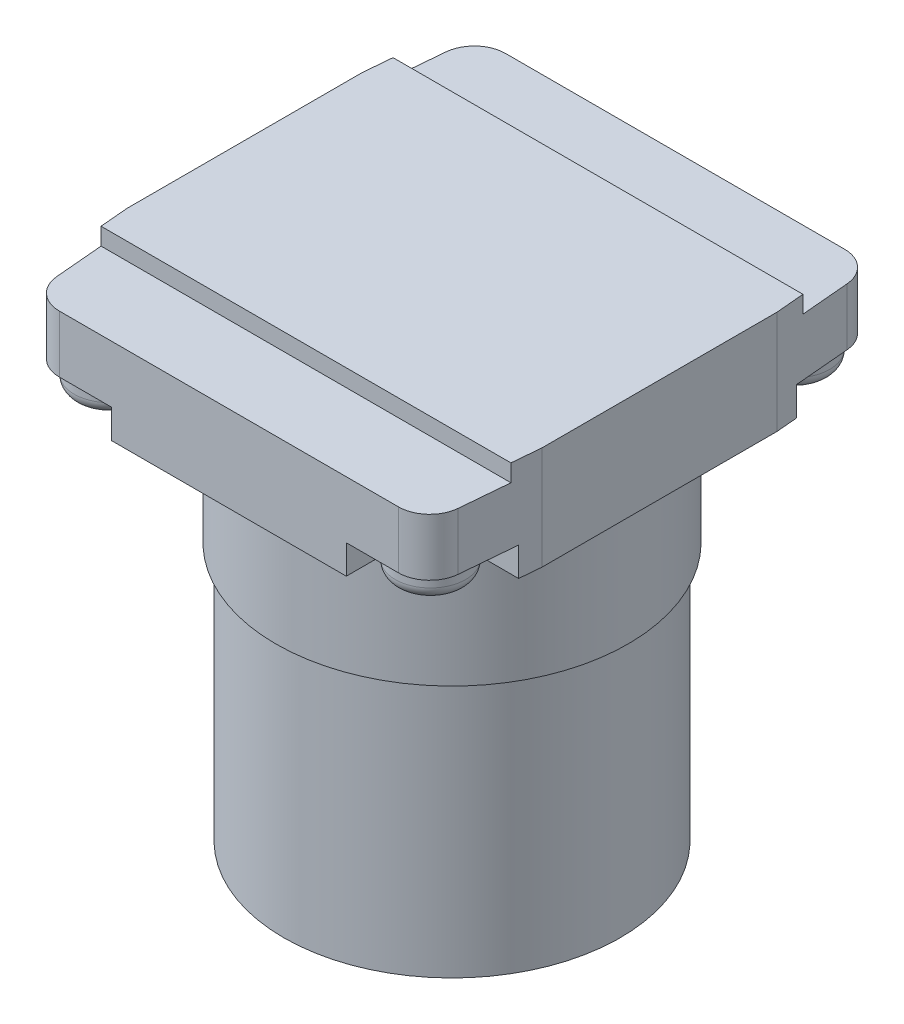
from build123d import *

# Parameters (mm, degrees)
EXTRUDE_1_DEPTH             = 26.5
EXTRUDE_1_DEPTH_BACK        = 26.5
SKETCH_2_W                  = 57
SKETCH_2_H                  = 61
CUT_EXTRUDE_1_DEPTH         = 32.5
EXTRUDE_2_DEPTH             = 2
SKETCH_5_W                  = 57
SKETCH_5_H                  = 61
CUT_EXTRUDE_2_DEPTH         = 3.7
PATTERN_LINEAR_1_COUNT      = 2
PATTERN_LINEAR_1_PITCH      = 46.5
PATTERN_LINEAR_1_COUNT_DIR2 = 2
PATTERN_LINEAR_1_PITCH_DIR2 = 41


with BuildPart() as part:
    # 草图1 → 凸台-拉伸1 (new, two sides: drawn at the far end of the back side and taken through both)
    with BuildSketch(Plane(origin=(0, 0, 0), x_dir=(0, 0, -1), z_dir=(1, 0, 0)).offset(-EXTRUDE_1_DEPTH_BACK)):
        Polygon((-28.5, -32.5), (28.5, -32.5), (28.5, -21.5), (18.65, -21.5), (18.65, -19.3), (-18.65, -19.3), (-18.65, -21.5), (-28.5, -21.5), align=None)
    extrude(amount=EXTRUDE_1_DEPTH + EXTRUDE_1_DEPTH_BACK)

    # 草图2 → 切除-拉伸1 (cut)
    with BuildSketch(Plane(origin=(0, 0, 0), x_dir=(1, 0, 0), z_dir=(0, 1, 0))):
        Rectangle(SKETCH_2_W, SKETCH_2_H)
        with BuildLine():
            Line((-26.5, -15), (-25.638357139, -24.848622971))
            ThreePointArc((-25.638357139, -24.848622971), (-24.355939177, -27.449109347), (-21.653578346, -28.5))
            Line((-21.653578346, -28.5), (21.653578346, -28.5))
            ThreePointArc((21.653578346, -28.5), (24.355939177, -27.449109347), (25.638357139, -24.848622971))
            Line((25.638357139, -24.848622971), (26.5, -15))
            Line((26.5, -15), (26.5, 15))
            Line((26.5, 15), (25.638357139, 24.848622971))
            ThreePointArc((25.638357139, 24.848622971), (24.355939177, 27.449109347), (21.653578346, 28.5))
            Line((21.653578346, 28.5), (-21.653578346, 28.5))
            ThreePointArc((-21.653578346, 28.5), (-24.355939177, 27.449109347), (-25.638357139, 24.848622971))
            Line((-25.638357139, 24.848622971), (-26.5, 15))
            Line((-26.5, 15), (-26.5, -15))
        make_face(mode=Mode.SUBTRACT)
    extrude(amount=-CUT_EXTRUDE_1_DEPTH, mode=Mode.SUBTRACT)

    # 草图3 → 旋转1 (revolve)
    with BuildSketch(Plane.XY, mode=Mode.PRIVATE) as revolve_1_sk:
        Polygon((0, -32.5), (22.5, -32.5), (22.5, -50.5), (21.5, -50.5), (21.5, -83.5), (0, -83.5), align=None)
    revolve(revolve_1_sk.sketch.rotate(Axis((0, -83.5, 0), (0, 1, 0)), 270), axis=Axis((0, -83.5, 0), (0, 1, 0)))

    # 草图4 → 凸台-拉伸2 (add)
    with BuildSketch(Plane(origin=(0, -32.5, 0), x_dir=(1, 0, 0), z_dir=(0, 1, 0))):
        with BuildLine():
            Line((-22.5, -2.9), (-19.5, -2.9))
            Line((-19.5, -2.9), (-19.5, 2.9))
            Line((-19.5, 2.9), (-22.5, 2.9))
            ThreePointArc((-22.5, 2.9), (-25.4, 0), (-22.5, -2.9))
        make_face()
    extrude(amount=-EXTRUDE_2_DEPTH)

    # 草图5 → 切除-拉伸2 (cut)
    with BuildSketch(Plane(origin=(0, -32.5, 0), x_dir=(1, 0, 0), z_dir=(0, 1, 0))):
        Rectangle(SKETCH_5_W, SKETCH_5_H)
        with BuildLine():
            Line((-26.5, -17.75), (-20.5, -17.75))
            ThreePointArc((-20.5, -17.75), (-16.610912703, -19.360912703), (-15, -23.25))
            Line((-15, -23.25), (-15, -28.5))
            Line((-15, -28.5), (15, -28.5))
            Line((15, -28.5), (15, -23.25))
            ThreePointArc((15, -23.25), (16.610912703, -19.360912703), (20.5, -17.75))
            Line((20.5, -17.75), (26.5, -17.75))
            Line((26.5, -17.75), (26.5, 17.75))
            Line((26.5, 17.75), (20.5, 17.75))
            ThreePointArc((20.5, 17.75), (16.610912703, 19.360912703), (15, 23.25))
            Line((15, 23.25), (15, 28.5))
            Line((15, 28.5), (-15, 28.5))
            Line((-15, 28.5), (-15, 23.25))
            ThreePointArc((-15, 23.25), (-16.610912703, 19.360912703), (-20.5, 17.75))
            Line((-20.5, 17.75), (-26.5, 17.75))
            Line((-26.5, 17.75), (-26.5, -17.75))
        make_face(mode=Mode.SUBTRACT)
    extrude(amount=CUT_EXTRUDE_2_DEPTH, mode=Mode.SUBTRACT)

    # 草图6 → 旋转2 (revolve)
    with BuildSketch(Plane.XY.offset(23.25), mode=Mode.PRIVATE) as revolve_2_sk:
        with BuildLine():
            Line((20.5, -28.8), (25, -28.8))
            Line((25, -28.8), (25, -30.5))
            ThreePointArc((25, -30.5), (24.53137085, -31.63137085), (23.4, -32.1))
            Line((23.4, -32.1), (20.5, -32.1))
            Line((20.5, -32.1), (20.5, -28.8))
        make_face()
    revolve_2 = revolve(revolve_2_sk.sketch.rotate(Axis((20.5, -32.1, 23.25), (0, 1, 0)), 270), axis=Axis((20.5, -32.1, 23.25), (0, 1, 0)))

    # 阵列(线性)1: Revolve 2 2 × 2
    with Locations(*[(-j * PATTERN_LINEAR_1_PITCH_DIR2, 0, -i * PATTERN_LINEAR_1_PITCH) for i in range(PATTERN_LINEAR_1_COUNT) for j in range(PATTERN_LINEAR_1_COUNT_DIR2) if (i, j) != (0, 0)]):
        add(revolve_2)


solid = part.part
